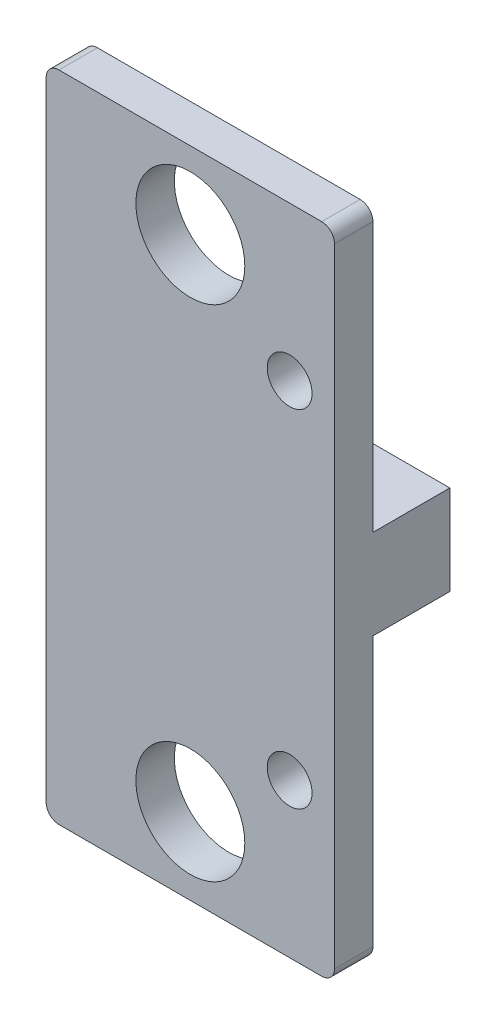
from build123d import *

# Parameters (mm, degrees)
SKETCH_1_W      = 45
SKETCH_1_H      = 58
SKETCH_1_R      = 8.5
EXTRUDE_1_DEPTH = 6
SKETCH_2_W      = 45
SKETCH_2_H      = 14
EXTRUDE_2_DEPTH = 12
M8X1_0_1_D      = 7
FILLET_1_R      = 2


with BuildPart() as part:
    # 草图1 → 凸台-拉伸1 (new body)
    with BuildSketch(Plane.XY):
        with Locations((0, -17)):
            Rectangle(SKETCH_1_W, SKETCH_1_H)
        Circle(SKETCH_1_R, mode=Mode.SUBTRACT)
    extrude_1 = extrude(amount=EXTRUDE_1_DEPTH)

    # 草图2 → 凸台-拉伸2 (add)
    with BuildSketch(Plane(origin=(0, 0, 0), x_dir=(-1, 0, 0), z_dir=(0, 0, -1))):
        with Locations((0, -39)):
            Rectangle(SKETCH_2_W, SKETCH_2_H)
    extrude(amount=EXTRUDE_2_DEPTH)

    # M8x1.0 螺纹孔1 (through all)
    with Locations(Plane(origin=(15.5, -12, 6), x_dir=(1, 0, 0), z_dir=(0, 0, 1))):
        with Locations((0, 0)):
            m8x1_0_1 = Hole(M8X1_0_1_D / 2)

    # 镜向1: 凸台-拉伸1, M8x1.0 螺纹孔1 across plane
    add(extrude_1.mirror(Plane(origin=(0, -39, 0), x_dir=(0, 0, 1), z_dir=(0, -1, 0))))
    add(m8x1_0_1.mirror(Plane(origin=(0, -39, 0), x_dir=(0, 0, 1), z_dir=(0, -1, 0))), mode=Mode.SUBTRACT)

    # 圆角1
    fillet_1_edges = [part.edges().sort_by_distance(p)[0] for p in [
        (22.5, -90, 3),
        (-22.5, -90, 3),
        (-22.5, 12, 3),
        (22.5, 12, 3),
    ]]
    fillet(fillet_1_edges, radius=FILLET_1_R)


solid = part.part
